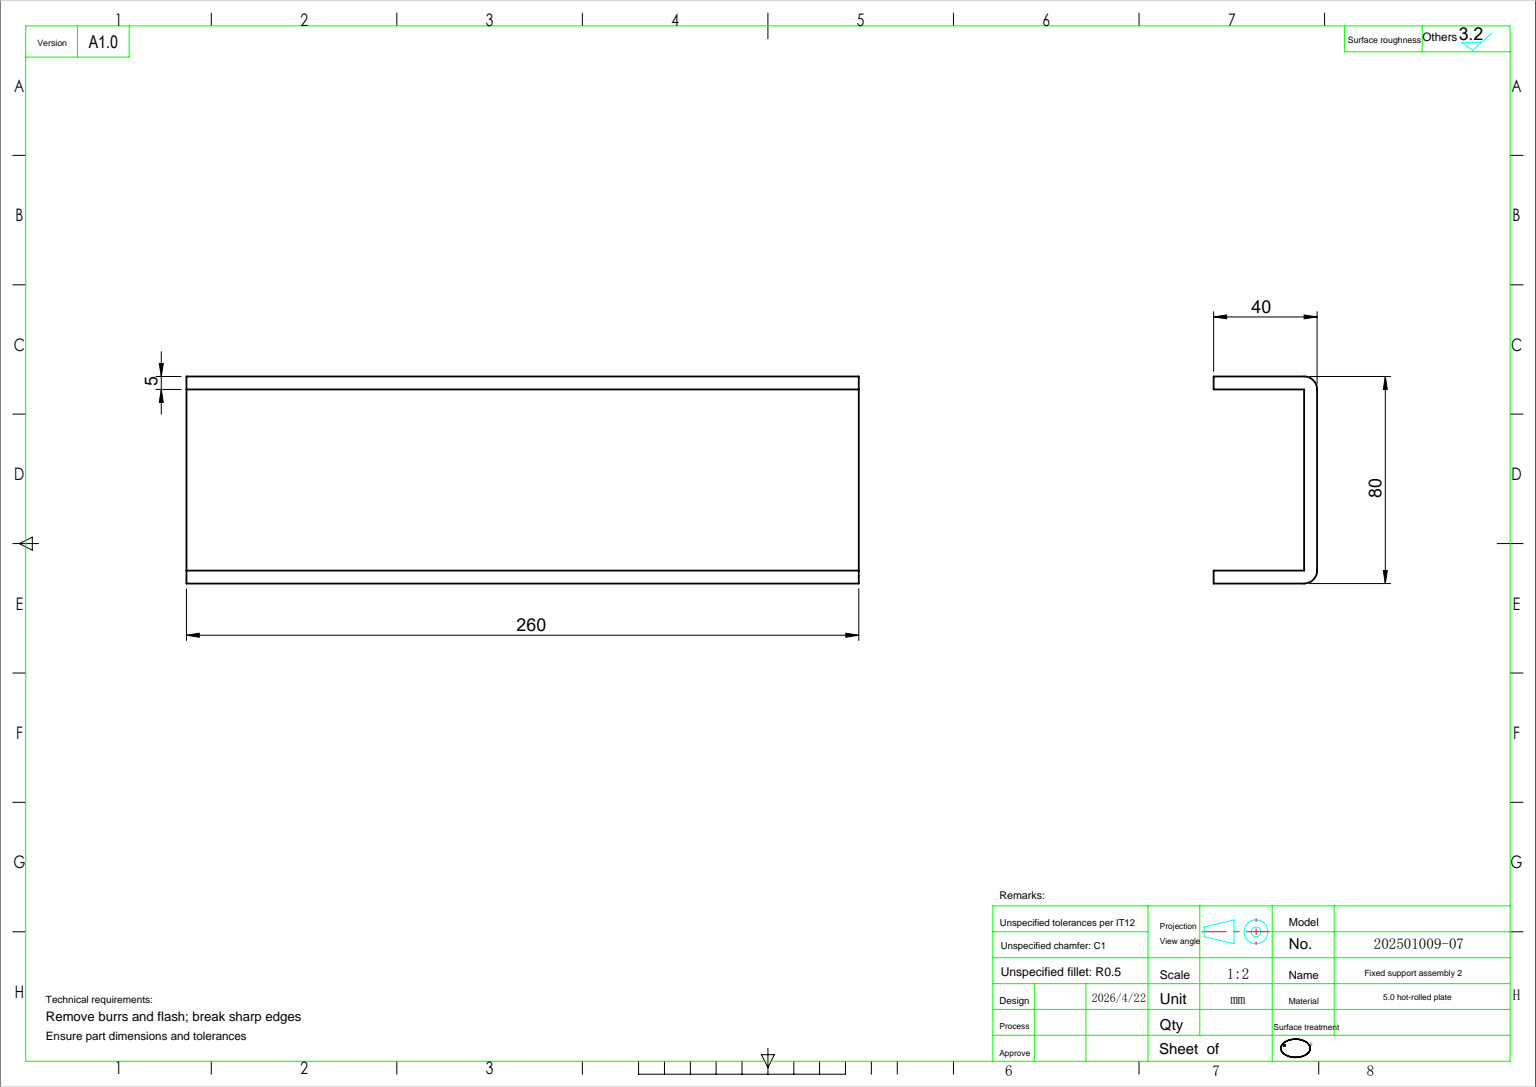
from build123d import *

# Parameters (mm, degrees)
EXTRUDE_1_DEPTH = 260
FILLET_1_R      = 5


with BuildPart() as part:
    # 草图1 → 拉伸-薄壁1 (new body)
    with BuildSketch(Plane.XY):
        Polygon((40, 40), (0, 40), (0, -40), (40, -40), (40, -35), (5, -35), (5, 35), (40, 35), align=None)
    extrude(amount=EXTRUDE_1_DEPTH)

    # 圆角1
    fillet_1_edges = [part.edges().sort_by_distance(p)[0] for p in [
        (0, -40, 130),
        (0, 40, 130),
    ]]
    fillet(fillet_1_edges, radius=FILLET_1_R)


solid = part.part
